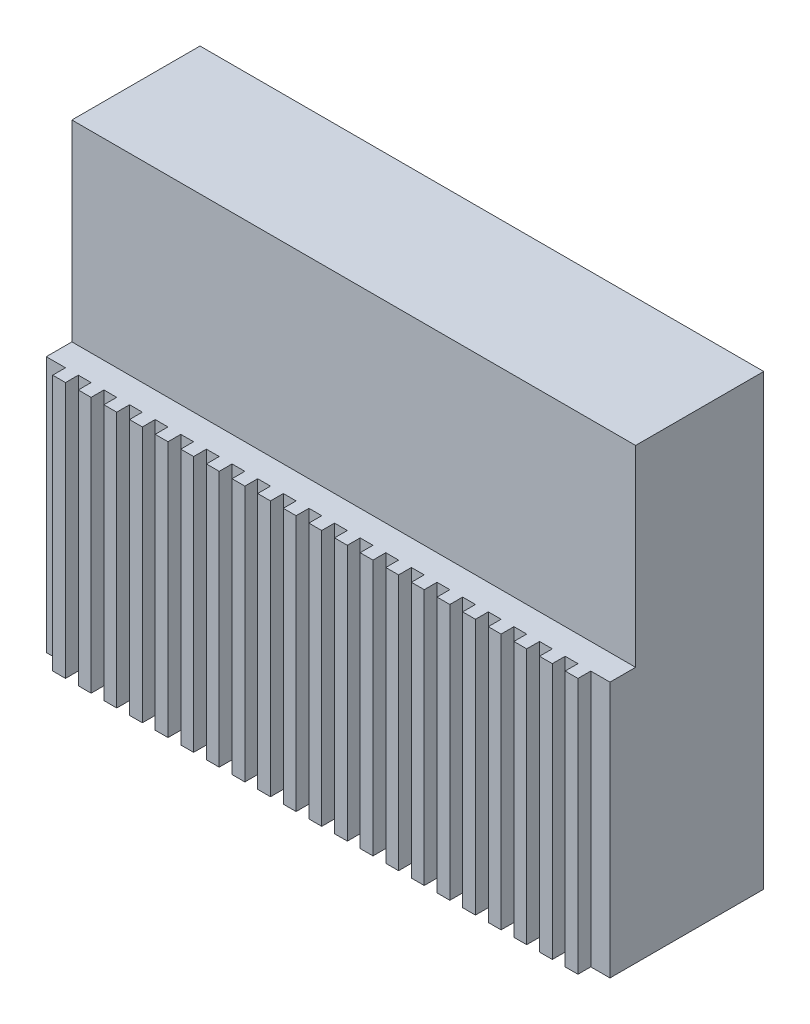
from build123d import *

# Parameters (mm, degrees)
SKETCH_1_W                = 44
SKETCH_1_H                = 35
EXTRUDE_1_DEPTH           = 10
SKETCH_2_W                = 44
SKETCH_2_H                = 20
EXTRUDE_2_DEPTH           = 2
SKETCH_4_W                = 1
SKETCH_4_H                = 20
EXTRUDE_3_DEPTH           = 1
PATTERN_LINEAR_1_COUNT    = 11
PATTERN_LINEAR_1_PITCH    = 2
MIRROR_1_COPY_1_SKETCH_W  = 1
MIRROR_1_COPY_1_SKETCH_H  = 20
MIRROR_1_COPY_1_DEPTH     = 1
MIRROR_1_COPY_2_SKETCH_W  = 1
MIRROR_1_COPY_2_SKETCH_H  = 20
MIRROR_1_COPY_2_DEPTH     = 1
MIRROR_1_COPY_3_SKETCH_W  = 1
MIRROR_1_COPY_3_SKETCH_H  = 20
MIRROR_1_COPY_3_DEPTH     = 1
MIRROR_1_COPY_4_SKETCH_W  = 1
MIRROR_1_COPY_4_SKETCH_H  = 20
MIRROR_1_COPY_4_DEPTH     = 1
MIRROR_1_COPY_5_SKETCH_W  = 1
MIRROR_1_COPY_5_SKETCH_H  = 20
MIRROR_1_COPY_5_DEPTH     = 1
MIRROR_1_COPY_6_SKETCH_W  = 1
MIRROR_1_COPY_6_SKETCH_H  = 20
MIRROR_1_COPY_6_DEPTH     = 1
MIRROR_1_COPY_7_SKETCH_W  = 1
MIRROR_1_COPY_7_SKETCH_H  = 20
MIRROR_1_COPY_7_DEPTH     = 1
MIRROR_1_COPY_8_SKETCH_W  = 1
MIRROR_1_COPY_8_SKETCH_H  = 20
MIRROR_1_COPY_8_DEPTH     = 1
MIRROR_1_COPY_9_SKETCH_W  = 1
MIRROR_1_COPY_9_SKETCH_H  = 20
MIRROR_1_COPY_9_DEPTH     = 1
MIRROR_1_COPY_10_SKETCH_W = 1
MIRROR_1_COPY_10_SKETCH_H = 20
MIRROR_1_COPY_10_DEPTH    = 1
MIRROR_1_COPY_11_SKETCH_W = 1
MIRROR_1_COPY_11_SKETCH_H = 20
MIRROR_1_COPY_11_DEPTH    = 1


with BuildPart() as part:
    # 草图1 → 凸台-拉伸1 (new body)
    with BuildSketch(Plane.XY):
        Rectangle(SKETCH_1_W, SKETCH_1_H)
    extrude(amount=EXTRUDE_1_DEPTH)

    # 草图2 → 凸台-拉伸2 (add)
    with BuildSketch(Plane.XY.offset(10)):
        with Locations((0, -7.5)):
            Rectangle(SKETCH_2_W, SKETCH_2_H)
    extrude(amount=EXTRUDE_2_DEPTH)

    # 草图4 → 凸台-拉伸3 (add)
    with BuildSketch(Plane.XY.offset(12)):
        with Locations((0, -7.5)):
            Rectangle(SKETCH_4_W, SKETCH_4_H)
    extrude_3 = extrude(amount=EXTRUDE_3_DEPTH)

    # 阵列(线性)1: 凸台-拉伸3 ×11
    with Locations(*[(i * PATTERN_LINEAR_1_PITCH, 0, 0) for i in range(1, PATTERN_LINEAR_1_COUNT)]):
        add(extrude_3)

    # 镜向1 copy 1 sketch → 镜向1 copy 1 (add)
    with BuildSketch(Plane(origin=(-2, 0, 12), x_dir=(-1, 0, 0), z_dir=(0, 0, 1))):
        with Locations((0, 7.5)):
            Rectangle(MIRROR_1_COPY_1_SKETCH_W, MIRROR_1_COPY_1_SKETCH_H)
    extrude(amount=MIRROR_1_COPY_1_DEPTH)

    # 镜向1 copy 2 sketch → 镜向1 copy 2 (add)
    with BuildSketch(Plane(origin=(-4, 0, 12), x_dir=(-1, 0, 0), z_dir=(0, 0, 1))):
        with Locations((0, 7.5)):
            Rectangle(MIRROR_1_COPY_2_SKETCH_W, MIRROR_1_COPY_2_SKETCH_H)
    extrude(amount=MIRROR_1_COPY_2_DEPTH)

    # 镜向1 copy 3 sketch → 镜向1 copy 3 (add)
    with BuildSketch(Plane(origin=(-6, 0, 12), x_dir=(-1, 0, 0), z_dir=(0, 0, 1))):
        with Locations((0, 7.5)):
            Rectangle(MIRROR_1_COPY_3_SKETCH_W, MIRROR_1_COPY_3_SKETCH_H)
    extrude(amount=MIRROR_1_COPY_3_DEPTH)

    # 镜向1 copy 4 sketch → 镜向1 copy 4 (add)
    with BuildSketch(Plane(origin=(-8, 0, 12), x_dir=(-1, 0, 0), z_dir=(0, 0, 1))):
        with Locations((0, 7.5)):
            Rectangle(MIRROR_1_COPY_4_SKETCH_W, MIRROR_1_COPY_4_SKETCH_H)
    extrude(amount=MIRROR_1_COPY_4_DEPTH)

    # 镜向1 copy 5 sketch → 镜向1 copy 5 (add)
    with BuildSketch(Plane(origin=(-10, 0, 12), x_dir=(-1, 0, 0), z_dir=(0, 0, 1))):
        with Locations((0, 7.5)):
            Rectangle(MIRROR_1_COPY_5_SKETCH_W, MIRROR_1_COPY_5_SKETCH_H)
    extrude(amount=MIRROR_1_COPY_5_DEPTH)

    # 镜向1 copy 6 sketch → 镜向1 copy 6 (add)
    with BuildSketch(Plane(origin=(-12, 0, 12), x_dir=(-1, 0, 0), z_dir=(0, 0, 1))):
        with Locations((0, 7.5)):
            Rectangle(MIRROR_1_COPY_6_SKETCH_W, MIRROR_1_COPY_6_SKETCH_H)
    extrude(amount=MIRROR_1_COPY_6_DEPTH)

    # 镜向1 copy 7 sketch → 镜向1 copy 7 (add)
    with BuildSketch(Plane(origin=(-14, 0, 12), x_dir=(-1, 0, 0), z_dir=(0, 0, 1))):
        with Locations((0, 7.5)):
            Rectangle(MIRROR_1_COPY_7_SKETCH_W, MIRROR_1_COPY_7_SKETCH_H)
    extrude(amount=MIRROR_1_COPY_7_DEPTH)

    # 镜向1 copy 8 sketch → 镜向1 copy 8 (add)
    with BuildSketch(Plane(origin=(-16, 0, 12), x_dir=(-1, 0, 0), z_dir=(0, 0, 1))):
        with Locations((0, 7.5)):
            Rectangle(MIRROR_1_COPY_8_SKETCH_W, MIRROR_1_COPY_8_SKETCH_H)
    extrude(amount=MIRROR_1_COPY_8_DEPTH)

    # 镜向1 copy 9 sketch → 镜向1 copy 9 (add)
    with BuildSketch(Plane(origin=(-18, 0, 12), x_dir=(-1, 0, 0), z_dir=(0, 0, 1))):
        with Locations((0, 7.5)):
            Rectangle(MIRROR_1_COPY_9_SKETCH_W, MIRROR_1_COPY_9_SKETCH_H)
    extrude(amount=MIRROR_1_COPY_9_DEPTH)

    # 镜向1 copy 10 sketch → 镜向1 copy 10 (add)
    with BuildSketch(Plane(origin=(-20, 0, 12), x_dir=(-1, 0, 0), z_dir=(0, 0, 1))):
        with Locations((0, 7.5)):
            Rectangle(MIRROR_1_COPY_10_SKETCH_W, MIRROR_1_COPY_10_SKETCH_H)
    extrude(amount=MIRROR_1_COPY_10_DEPTH)

    # 镜向1 copy 11 sketch → 镜向1 copy 11 (add)
    with BuildSketch(Plane(origin=(0, 0, 12), x_dir=(-1, 0, 0), z_dir=(0, 0, 1))):
        with Locations((0, 7.5)):
            Rectangle(MIRROR_1_COPY_11_SKETCH_W, MIRROR_1_COPY_11_SKETCH_H)
    extrude(amount=MIRROR_1_COPY_11_DEPTH)


solid = part.part
